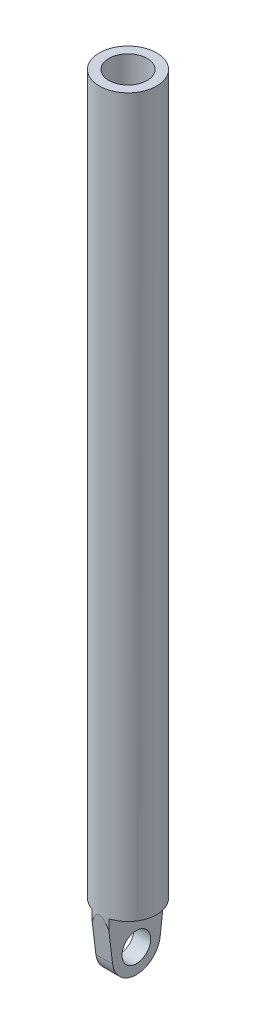
from build123d import *
from build123d.topology import SkipClean

# Parameters (mm, degrees)
SKETCH1_R           = 6
BOSS_EXTRUDE1_DEPTH = 150
SHELL1_T            = -2
SKETCH2_R           = 3
BOSS_EXTRUDE2_DEPTH = 1.75
CUT_EXTRUDE1_START  = 10
SKETCH3_R           = 8.578209266
SKETCH3_R_2         = 6
CUT_EXTRUDE1_DEPTH  = 10


with BuildPart() as part:
    # Sketch1 → Boss-Extrude1 (new body)
    with BuildSketch(Plane(origin=(0, 0, 0), x_dir=(1, 0, 0), z_dir=(0, 1, 0))):
        with Locations(Location((0, 0, 0), (0, 0, 270))):
            Circle(SKETCH1_R)
    extrude(amount=BOSS_EXTRUDE1_DEPTH)

    # Shell1
    shell1_openings = [part.faces().sort_by_distance(p)[0] for p in [
        (0, 150, 0),
    ]]
    offset(amount=SHELL1_T, openings=shell1_openings, kind=Kind.INTERSECTION)

    # Sketch2 → Boss-Extrude2 (add, symmetric)
    with BuildSketch(Plane(origin=(0, 0, 0), x_dir=(0, 0, -1), z_dir=(1, 0, 0))):
        with BuildLine():
            Line((-6, 0), (6, 0))
            Line((6, 0), (4.964101615, -8.598076211))
            ThreePointArc((4.964101615, -8.598076211), (0, -13), (-4.964101615, -8.598076211))
            Line((-4.964101615, -8.598076211), (-6, 0))
        make_face()
        with Locations((0, -8)):
            Circle(SKETCH2_R, mode=Mode.SUBTRACT)
    extrude(amount=BOSS_EXTRUDE2_DEPTH, both=True)

    # Sketch3 → Cut-Extrude1 (cut)
    with SkipClean():  # the faces are left unmerged after this step: merging them gives an invalid solid
        with BuildSketch(Plane.XZ.offset(CUT_EXTRUDE1_START)):
            Circle(SKETCH3_R)
            with Locations(Location((0, 0, 0), (0, 0, 253.0422367))):
                Circle(SKETCH3_R_2, mode=Mode.SUBTRACT)
        extrude(amount=-CUT_EXTRUDE1_DEPTH, mode=Mode.SUBTRACT)


solid = part.part
